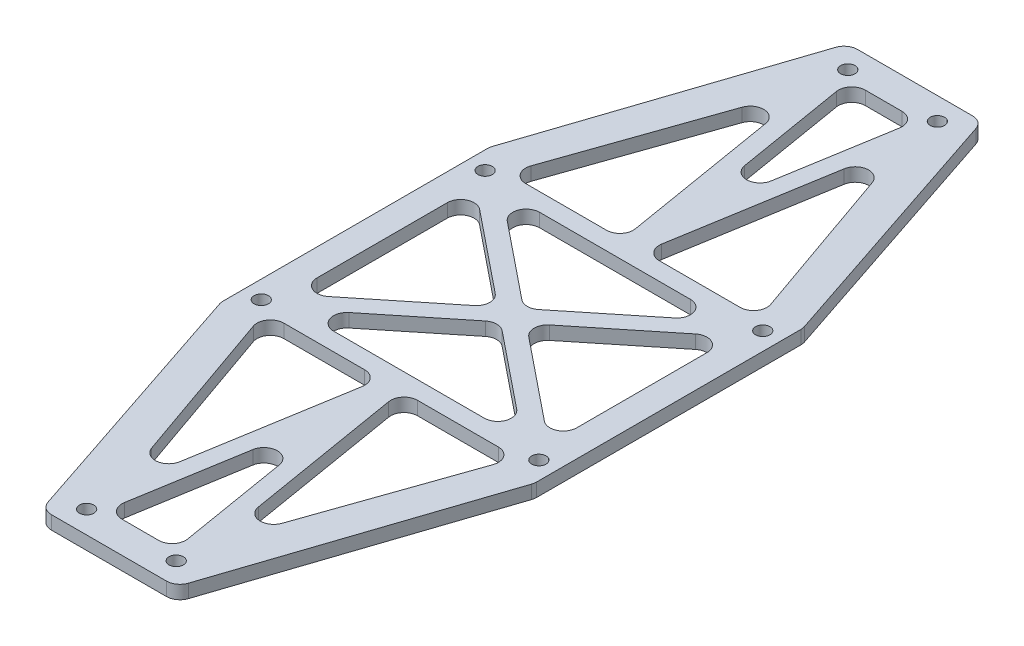
SolidWorks part; units mm, degrees
material "哈碳纤"
ref_plane "前视基准面" through (0, 0, 0) normal (0, 0, 1) x (1, 0, 0)
ref_plane "上视基准面" through (0, 0, 0) normal (0, 1, 0) x (1, 0, 0)
ref_plane "右视基准面" through (0, 0, 0) normal (1, 0, 0) x (0, 0, -1)
other "Configuration Table"
sketch "草图1" plane through (0, 0, 0) normal (0, 1, 0) x (1, 0, 0)
  line L0 (-15, 90) -> (-35, 30)
  line L1 (-35, 30) -> (-35, -30)
  line L2 (-35, -30) -> (-15, -90)
  line L3 (-15, -90) -> (15, -90)
  line L4 (15, -90) -> (35, -30)
  line L5 (35, -30) -> (35, 30)
  line L6 (35, 30) -> (15, 90)
  line L7 (15, 90) -> (-15, 90)
  line L8 (-35, 30) -> (35, -30) construction
  line L9 (35, 30) -> (-35, -30) construction
  line L10 (-35, 30) -> (35, 30) construction
  line L11 (-35, -30) -> (35, -30) construction
  line L12 (-15, 90) -> (0, 30) construction
  line L13 (15, 90) -> (0, 30) construction
  point P2 (0, 0)
  point P9 (0, 90)
  point P11 (0, -90)
  point P12 (35, 0)
  dimension "D1" = 180
  dimension "D2" = 70
  dimension "D3" = 60
  dimension "D4" = 30
extrude "凸台-拉伸1" add sketch "草图1" along normal blind 3
sketch "草图2" plane through (0, 3, 0) normal (0, 1, 0) x (1, 0, 0)
  line L0 (15, 90) -> (-15, 90) construction
  line L1 (-31, -25) -> (31, -25) construction
  line L2 (-31, -25) -> (-31, 25) construction
  line L3 (-31, 25) -> (31, 25) construction
  line L4 (31, -25) -> (31, 25) construction
  line L5 (-31, -25) -> (31, 25) construction
  line L6 (-31, 25) -> (31, -25) construction
  line L7 (-10, 85) -> (10, 85) construction
  line L8 (-1000, 0) -> (49000, 0) construction
  line L9 (-10, -85) -> (10, -85) construction
  circle A0 centre (-31, 25) radius 1.6
  circle A1 centre (31, 25) radius 1.6
  circle A2 centre (31, -25) radius 1.6
  circle A3 centre (-31, -25) radius 1.6
  circle A4 centre (-10, 85) radius 1.6
  circle A5 centre (10, 85) radius 1.6
  circle A6 centre (10, -85) radius 1.6
  circle A7 centre (-10, -85) radius 1.6
  point P0 (0, 0)
  point P16 (0, 85)
  dimension "D3" = 3.2
  dimension "D4" = 3.2
  dimension "D5" = 3.2
  dimension "D1" = 50
  dimension "D2" = 62
  dimension "D6" = 20
  dimension "D7" = 5
extrude "切除-拉伸1" cut sketch "草图2" against normal blind 3
sketch "草图4" plane through (0, 3, 0) normal (0, 1, 0) x (1, 0, 0)
  line L0 (-31, 25) -> (-10, 85) construction
  line L1 (-31, -25) -> (31, -25) construction
  line L2 (-31, -25) -> (-31, 25) construction
  line L3 (-31, 25) -> (31, 25) construction
  line L4 (31, -25) -> (31, 25) construction
  line L5 (-31, -25) -> (31, 25) construction
  line L6 (-31, 25) -> (31, -25) construction
  line L7 (-10, 85) -> (0, 25) construction
  line L8 (0, 25) -> (10, 85) construction
  line L9 (10, 85) -> (31, 25) construction
  line L10 (-29.1123, 24.3393) -> (-10.69, 76.9744)
  line L11 (-10.69, 76.9744) -> (0, 12.8345)
  line L12 (0, 12.8345) -> (10.69, 76.9744)
  line L13 (10.69, 76.9744) -> (29.1123, 24.3393)
  line L14 (-31, -27) -> (31, -27)
  line L15 (-29, -25) -> (-29, 25)
  line L16 (-31, 23) -> (31, 23)
  line L17 (33, -25) -> (33, 25)
  line L18 (-29.7445, -26.5568) -> (32.2555, 23.4432)
  line L19 (-32.2555, 23.4432) -> (29.7445, -26.5568)
  line L20 (-32.8877, 25.6607) -> (-9.31, 93.0256)
  line L21 (-9.31, 93.0256) -> (0, 37.1655)
  line L22 (0, 37.1655) -> (9.31, 93.0256)
  line L23 (9.31, 93.0256) -> (32.8877, 25.6607)
  line L24 (-31, -23) -> (31, -23)
  line L25 (-33, -25) -> (-33, 25)
  line L26 (-31, 27) -> (31, 27)
  line L27 (29, -25) -> (29, 25)
  line L28 (-32.2555, -23.4432) -> (29.7445, 26.5568)
  line L29 (-29.7445, 26.5568) -> (32.2555, -23.4432)
  line L30 (-1000, 0) -> (49000, 0) construction
  line L31 (-10, 85) -> (10, 85) construction
  line L32 (-10, 83) -> (10, 83)
  line L33 (-10, 87) -> (10, 87)
  line L34 (0, -25) -> (10, -85) construction
  line L35 (10, -85) -> (31, -25) construction
  line L36 (-10, -85) -> (10, -85) construction
  line L37 (-10, -85) -> (0, -25) construction
  line L38 (-31, -25) -> (-10, -85) construction
  line L39 (-8.0272, -85.3288) -> (0, -37.1655)
  line L40 (0, -37.1655) -> (8.0272, -85.3288)
  line L41 (11.8877, -85.6607) -> (32.8877, -25.6607)
  line L42 (-10, -87) -> (10, -87)
  line L43 (-32.8877, -25.6607) -> (-11.8877, -85.6607)
  line L44 (-11.9728, -84.6712) -> (0, -12.8345)
  line L45 (0, -12.8345) -> (11.9728, -84.6712)
  line L46 (8.1123, -84.3393) -> (29.1123, -24.3393)
  line L47 (-10, -83) -> (10, -83)
  line L48 (-29.1123, -24.3393) -> (-8.1123, -84.3393)
  point P0 (0, 0)
  dimension "D1" = 2
  dimension "D2" = 2
  dimension "D3" = 2
  dimension "D4" = 2
  dimension "D5" = 2
  dimension "D6" = 2
extrude "切除-拉伸2" cut sketch "草图4" against normal blind 3 contours L10 L26 L11 | L12 L26 L13 | L32 L21 L22 | L16 L29 L28 L12 L11 | L16 L11 L12 | L15 L28 L19 | L18 L29 L27 | L44 L45 L24 L19 L18 | L45 L44 L24 | L14 L48 L44 | L45 L46 L14 | L39 L47 L40
fillet "圆角1" radius 3 38 edges at (-2.3609, 1.5, 27) (-10.69, 1.5, 76.9744) (-28.181, 1.5, 27) (0, 1.5, 2.5693) (25.334, 1.5, 23) (-25.334, 1.5, 23) (-25.334, 1.5, -23) (25.334, 1.5, -23) (0, 1.5, -2.5693) (10.69, 1.5, -76.9744) (28.181, 1.5, -27) (2.3609, 1.5, -27) (0, 1.5, 37.1655) (7.6391, 1.5, 83) (-7.6391, 1.5, 83) (-15, 1.5, -90) (-35, 1.5, -30) (-35, 1.5, 30) (-15, 1.5, 90) (15, 1.5, 90) (35, 1.5, 30) (35, 1.5, -30) (15, 1.5, -90) (-10.69, 1.5, -76.9744) (-2.3609, 1.5, -27) (-28.181, 1.5, -27) (7.6391, 1.5, -83) (0, 1.5, -37.1655) (-7.6391, 1.5, -83) (-3.186, 1.5, 0) (-29, 1.5, 20.8178) (29, 1.5, -20.8178) (29, 1.5, 20.8178) (3.186, 1.5, 0) (28.181, 1.5, 27) (10.69, 1.5, 76.9744) (2.3609, 1.5, 27) (-29, 1.5, -20.8178)
